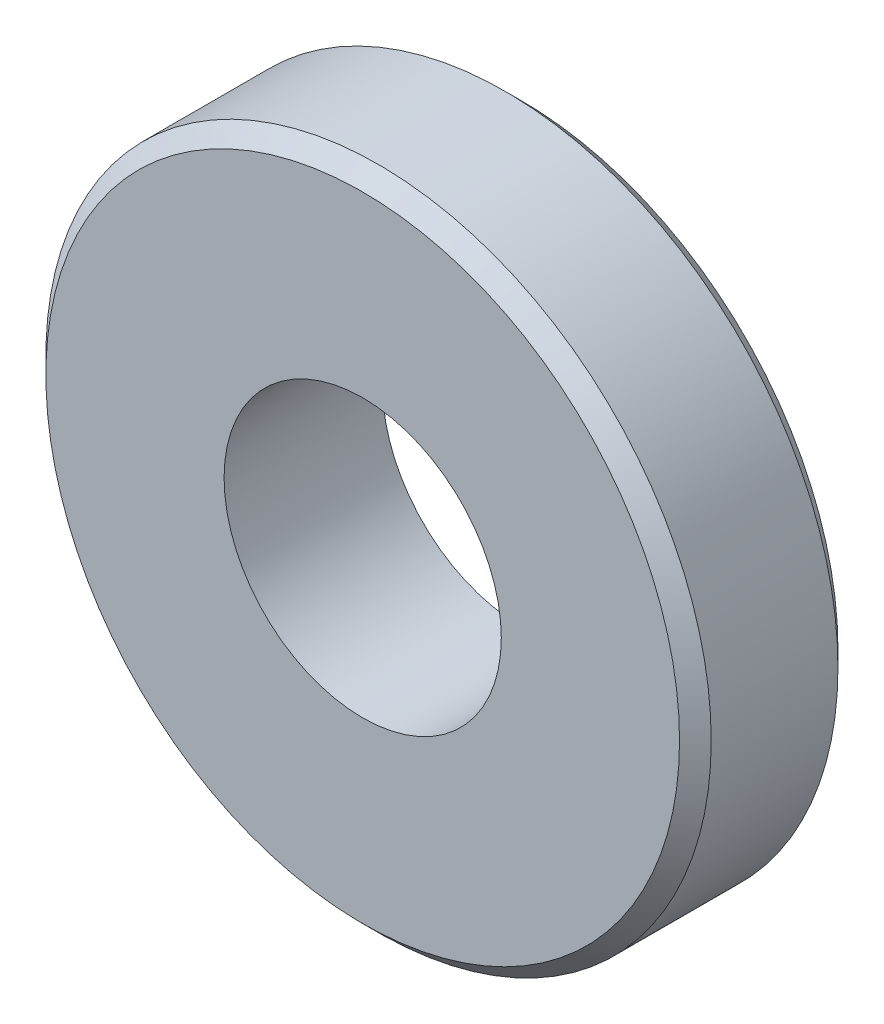
SolidWorks part; units mm, degrees
ref_plane "Front Plane" through (0, 0, 0) normal (0, 0, 1) x (1, 0, 0)
ref_plane "Top Plane" through (0, 0, 0) normal (0, 1, 0) x (1, 0, 0)
ref_plane "Right Plane" through (0, 0, 0) normal (1, 0, 0) x (0, 0, -1)
other "Configuration Table"
sketch "Sketch1" plane through (0, 0, 0) normal (0, 0, 1) x (1, 0, 0)
  circle A0 centre (0, 0) radius 210
  circle A1 centre (0, 0) radius 87.5
  dimension "D1" = 175
  dimension "D2" = 420
extrude "Boss-Extrude1" add sketch "Sketch1" along normal blind 100
chamfer "Chamfer1" distance 10 angle 45 2 edges at (210, 0, 0) (210, 0, 100)
